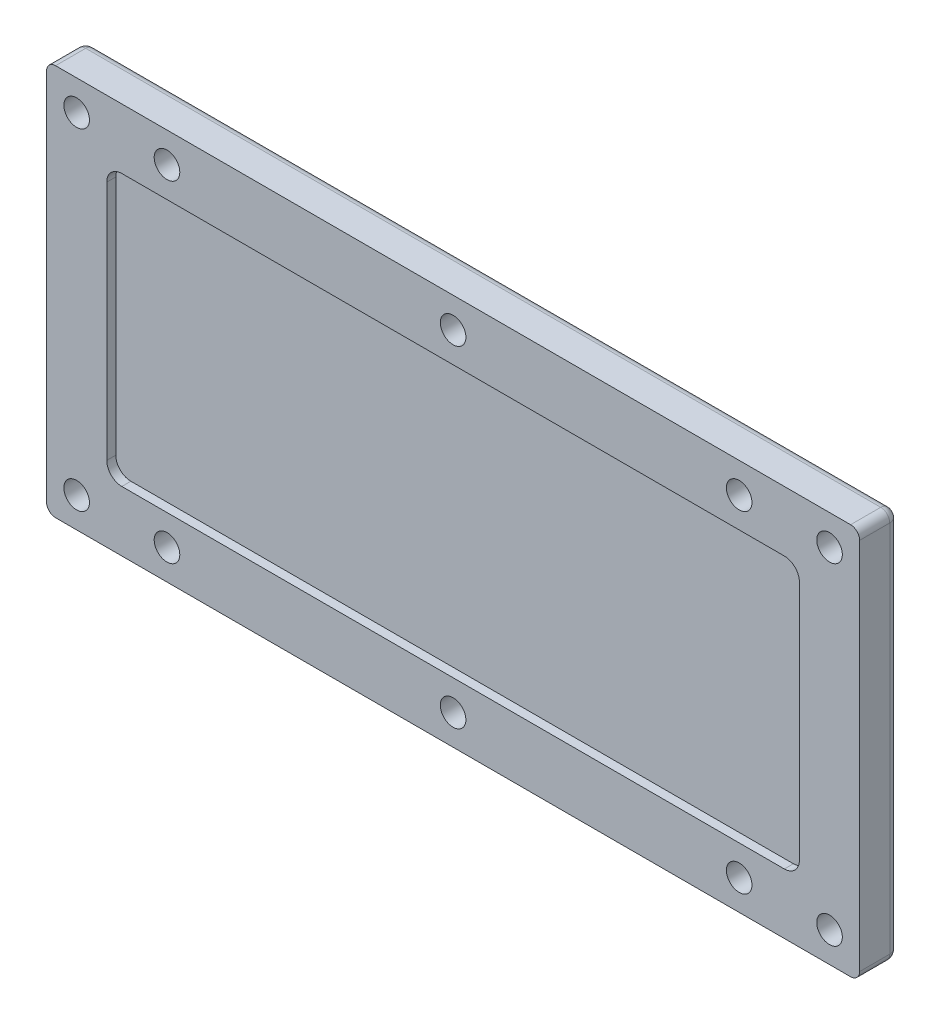
SolidWorks part; units mm, degrees
material "普通碳钢"
ref_plane "前视基准面" through (0, 0, 0) normal (0, 0, 1) x (1, 0, 0)
ref_plane "上视基准面" through (0, 0, 0) normal (0, 1, 0) x (1, 0, 0)
ref_plane "右视基准面" through (0, 0, 0) normal (1, 0, 0) x (0, 0, -1)
sketch "草图1" plane through (0, 0, 0) normal (0, 0, 1) x (1, 0, 0)
  line L0 (0, 0) -> (0, 55) construction
  line L1 (-132, -65) -> (132, -65)
  line L2 (-135, -62) -> (-135, 62)
  line L3 (-132, 65) -> (132, 65)
  line L4 (135, -62) -> (135, 62)
  line L5 (-135, -65) -> (135, 65) construction
  line L6 (-135, 65) -> (135, -65) construction
  line L7 (-125, -55) -> (125, -55) construction
  line L8 (-125, -55) -> (-125, 55) construction
  line L9 (-125, 55) -> (125, 55) construction
  line L10 (125, -55) -> (125, 55) construction
  line L11 (-125, -55) -> (125, 55) construction
  line L12 (-125, 55) -> (125, -55) construction
  line L13 (0, 0) -> (0, -55) construction
  line L14 (-95, 55) -> (-95, -55) construction
  line L15 (95, 55) -> (95, -55) construction
  arc A0 (132, 65) -> (135, 62) centre (132, 62) cw
  arc A1 (132, -65) -> (135, -62) centre (132, -62) ccw
  arc A2 (-132, -65) -> (-135, -62) centre (-132, -62) cw
  arc A3 (-135, 62) -> (-132, 65) centre (-132, 62) cw
  circle A4 centre (-125, 55) radius 4.25
  circle A5 centre (-95, 55) radius 4.25
  circle A6 centre (0, 55) radius 4.25
  circle A7 centre (95, 55) radius 4.25
  circle A8 centre (125, 55) radius 4.25
  circle A9 centre (125, -55) radius 4.25
  circle A10 centre (95, -55) radius 4.25
  circle A11 centre (0, -55) radius 4.25
  circle A12 centre (-95, -55) radius 4.25
  circle A13 centre (-125, -55) radius 4.25
  point P0 (0, 0)
  point P18 (0, 0)
  dimension "D3" = 3
  dimension "D8" = 8.5
  dimension "D1" = 270
  dimension "D2" = 130
  dimension "D4" = 250
  dimension "D5" = 110
  dimension "D6" = 95
  dimension "D7" = 95
extrude "凸台-拉伸1" add sketch "草图1" along normal blind 10
sketch "草图2" plane through (0, 0, 10) normal (0, 0, 1) x (1, 0, 0)
  line L1 (-110, -45) -> (110, -45)
  line L2 (-115, -40) -> (-115, 40)
  line L3 (-110, 45) -> (110, 45)
  line L4 (132, 65) -> (-132, 65)
  line L5 (-135, 62) -> (-135, -62)
  line L6 (-132, -65) -> (132, -65)
  line L7 (135, -62) -> (135, 62)
  line L8 (132, 65) -> (-132, 65)
  line L9 (-135, 62) -> (-135, -62)
  line L10 (-132, -65) -> (132, -65)
  line L11 (135, -62) -> (135, 62)
  line L12 (115, -40) -> (115, 40)
  line L13 (-115, -45) -> (115, 45) construction
  line L14 (-115, 45) -> (115, -45) construction
  circle A0 centre (-125, -55) radius 4.25 construction
  circle A1 centre (-95, -55) radius 4.25 construction
  circle A2 centre (0, -55) radius 4.25 construction
  circle A3 centre (95, -55) radius 4.25 construction
  arc A4 (135, 62) -> (132, 65) centre (132, 62) ccw
  arc A5 (-132, 65) -> (-135, 62) centre (-132, 62) ccw
  arc A6 (-135, -62) -> (-132, -65) centre (-132, -62) ccw
  arc A7 (132, -65) -> (135, -62) centre (132, -62) ccw
  arc A8 (135, 62) -> (132, 65) centre (132, 62) ccw
  arc A9 (-132, 65) -> (-135, 62) centre (-132, 62) ccw
  arc A10 (-135, -62) -> (-132, -65) centre (-132, -62) ccw
  arc A11 (132, -65) -> (135, -62) centre (132, -62) ccw
  circle A12 centre (125, -55) radius 4.25 construction
  circle A13 centre (125, 55) radius 4.25 construction
  circle A14 centre (95, 55) radius 4.25 construction
  circle A15 centre (0, 55) radius 4.25 construction
  circle A16 centre (-95, 55) radius 4.25 construction
  circle A17 centre (-125, 55) radius 4.25 construction
  circle A18 centre (-125, -55) radius 4.25
  circle A19 centre (-95, -55) radius 4.25
  circle A20 centre (0, -55) radius 4.25
  circle A21 centre (95, -55) radius 4.25
  circle A22 centre (125, -55) radius 4.25
  circle A23 centre (125, 55) radius 4.25
  circle A24 centre (95, 55) radius 4.25
  circle A25 centre (0, 55) radius 4.25
  circle A26 centre (-95, 55) radius 4.25
  circle A27 centre (-125, 55) radius 4.25
  arc A28 (110, 45) -> (115, 40) centre (110, 40) cw
  arc A29 (110, -45) -> (115, -40) centre (110, -40) ccw
  arc A30 (-115, -40) -> (-110, -45) centre (-110, -40) ccw
  arc A31 (-115, 40) -> (-110, 45) centre (-110, 40) cw
  point P42 (0, 0)
  dimension "D4" = 5
  dimension "D2" = 230
  dimension "D3" = 90
  dimension "D1" = 0
extrude "凸台-拉伸2" add sketch "草图2" along normal blind 3
fillet "圆角1" radius 3 8 edges at (134.1213, -64.1213, 0) (0, -65, 0) (-134.1213, -64.1213, 0) (-135, 0, 0) (-134.1213, 64.1213, 0) (0, 65, 0) (134.1213, 64.1213, 0) (135, 0, 0)
